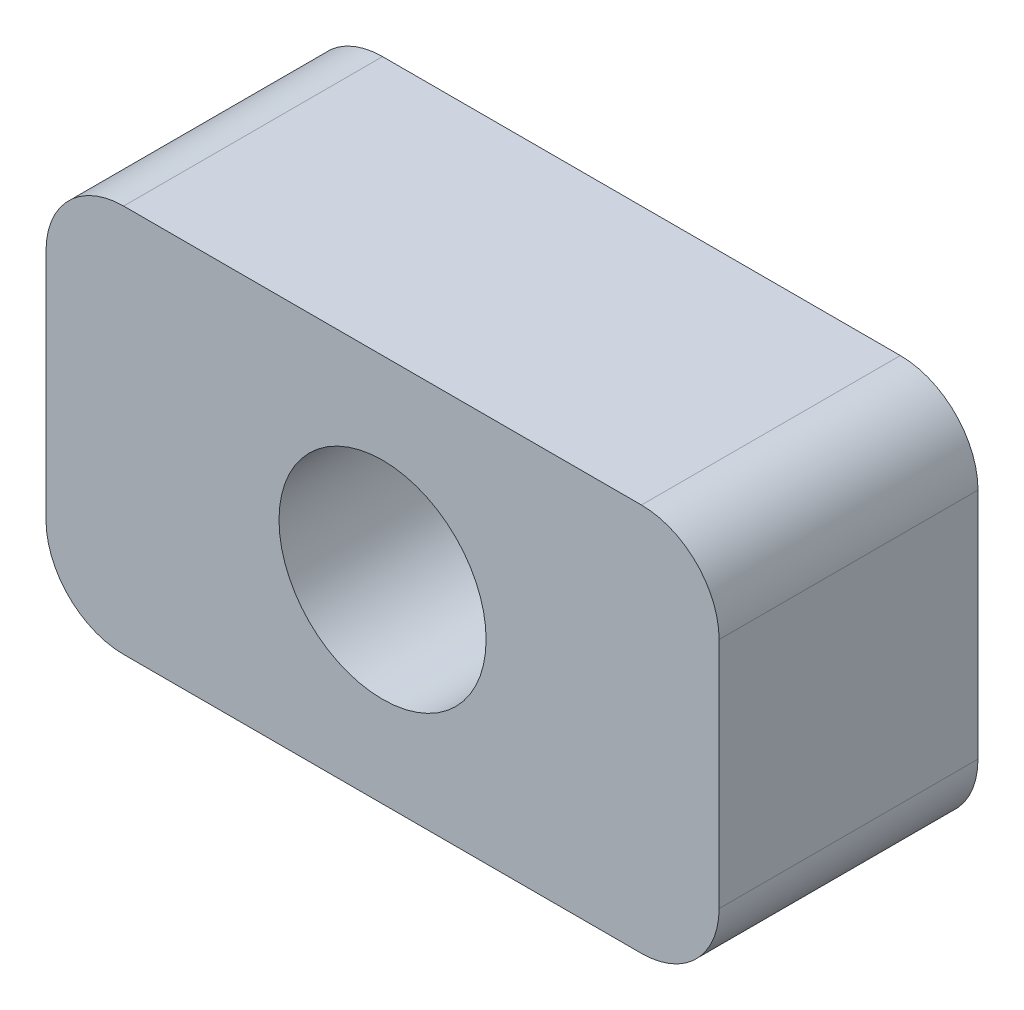
SolidWorks part; units mm, degrees
ref_plane "Front Plane" through (0, 0, 0) normal (0, 0, 1) x (1, 0, 0)
ref_plane "Top Plane" through (0, 0, 0) normal (0, 1, 0) x (1, 0, 0)
ref_plane "Right Plane" through (0, 0, 0) normal (1, 0, 0) x (0, 0, -1)
sketch "Sketch1" plane through (0, 0, 0) normal (0, 0, 1) x (1, 0, 0)
  line L1 (-13, 7.5) -> (13, 7.5)
  line L2 (-13, 7.5) -> (-13, -7.5)
  line L3 (-13, -7.5) -> (13, -7.5)
  line L4 (13, 7.5) -> (13, -7.5)
  line L5 (-13, 7.5) -> (13, -7.5) construction
  line L6 (-13, -7.5) -> (13, 7.5) construction
  circle A0 centre (0, 0) radius 4
  point P0 (0, 0)
  dimension "D3" = 8
  dimension "D1" = 26
  dimension "D2" = 15
extrude "Boss-Extrude1" add sketch "Sketch1" along normal blind 10
fillet "Fillet1" radius 3 4 edges at (-13, 7.5, 5) (-13, -7.5, 5) (13, -7.5, 5) (13, 7.5, 5)
